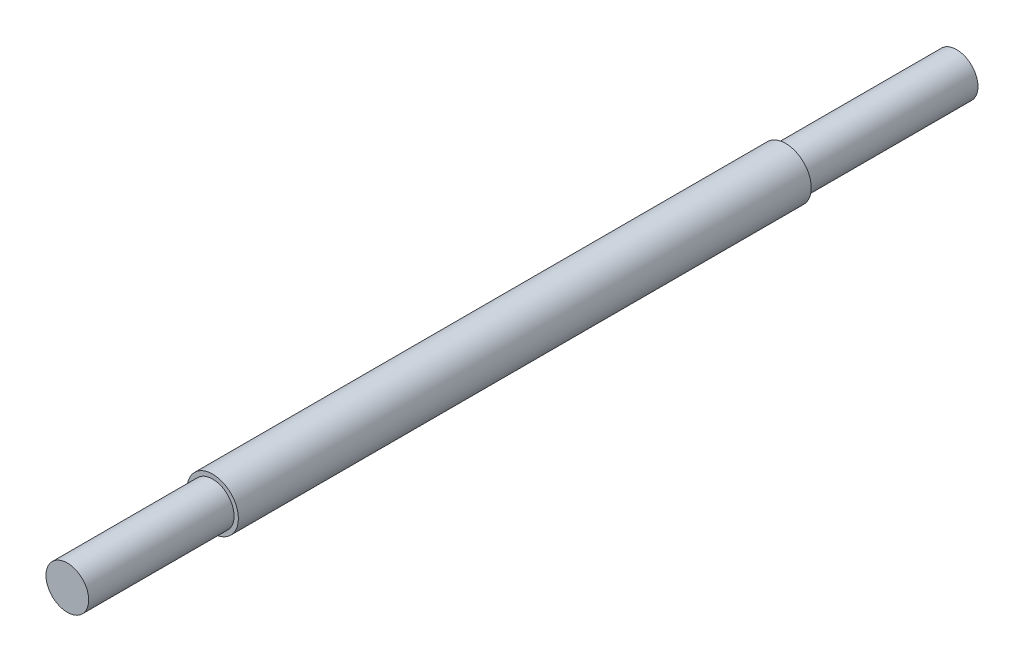
SolidWorks part; units mm, degrees
ref_plane "Front Plane" through (0, 0, 0) normal (0, 0, 1) x (1, 0, 0)
ref_plane "Top Plane" through (0, 0, 0) normal (0, 1, 0) x (1, 0, 0)
ref_plane "Right Plane" through (0, 0, 0) normal (1, 0, 0) x (0, 0, -1)
sketch "Sketch1" plane through (0, 0, 0) normal (0, 0, 1) x (1, 0, 0)
  circle A0 centre (0, 0) radius 2.5
extrude "Boss-Extrude1" add sketch "Sketch1" along normal blind 20
sketch "Sketch2" plane through (0, 0, 20) normal (0, 0, 1) x (1, 0, 0)
  circle A0 centre (0, 0) radius 3
extrude "Boss-Extrude2" add sketch "Sketch2" along normal blind 67
sketch "Sketch3" plane through (0, 0, 87) normal (0, 0, 1) x (1, 0, 0)
  circle A0 centre (0, 0) radius 2.5
extrude "Boss-Extrude3" add sketch "Sketch3" along normal blind 17
